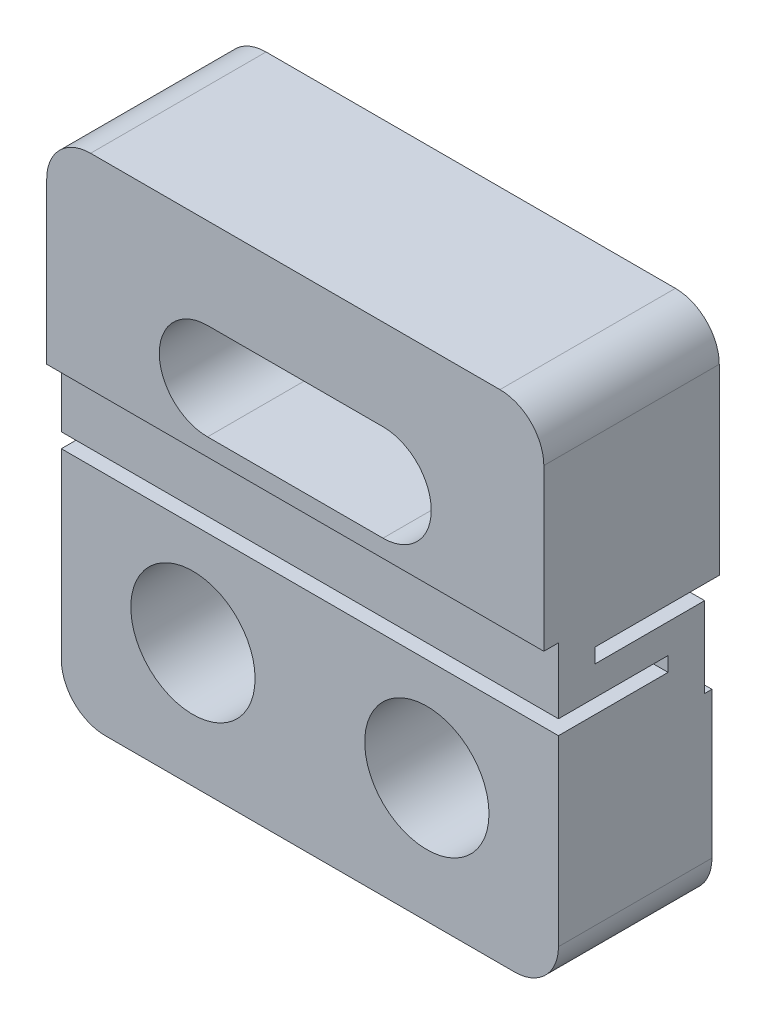
from build123d import *

# Parameters (mm, degrees)
SKETCH1_W           = 34
SKETCH1_H           = 35
BOSS_EXTRUDE1_DEPTH = 12
SKETCH2_R           = 2.1
CUT_EXTRUDE1_DEPTH  = 28.189152249
SKETCH3_W           = 43.383687714
SKETCH3_H           = 21.18675689
CUT_EXTRUDE2_DEPTH  = 1
SKETCH4_W           = 50.621361837
SKETCH4_H           = 17.880513978
CUT_EXTRUDE3_DEPTH  = 0.5
CUT_EXTRUDE4_DEPTH  = 1
SKETCH6_R           = 4.25
CUT_EXTRUDE5_DEPTH  = 6.5
SKETCH7_W           = 35.621240015
SKETCH7_H           = 1
CUT_EXTRUDE6_DEPTH  = 7.5
SKETCH8_W           = 34
SKETCH8_H           = 1
CUT_EXTRUDE7_DEPTH  = 7.5
FILLET1_R           = 3


with BuildPart() as part:
    # Sketch1 → Boss-Extrude1 (new body)
    with BuildSketch(Plane.XY):
        Rectangle(SKETCH1_W, SKETCH1_H)
    extrude(amount=BOSS_EXTRUDE1_DEPTH)

    # Sketch2 → Cut-Extrude1 (cut, through all)
    with BuildSketch(Plane.XY.offset(12)):
        with Locations((-8, -9)):
            Circle(SKETCH2_R)
        with Locations((8, -9)):
            Circle(SKETCH2_R)
        with BuildLine():
            Line((-6, 11.3), (6, 11.3))
            ThreePointArc((6, 11.3), (9.3, 8), (6, 4.7))
            Line((6, 4.7), (-6, 4.7))
            ThreePointArc((-6, 4.7), (-9.3, 8), (-6, 11.3))
        make_face()
    extrude(amount=-CUT_EXTRUDE1_DEPTH, mode=Mode.SUBTRACT)

    # Sketch3 → Cut-Extrude2 (cut)
    with BuildSketch(Plane.XY.offset(12)):
        with Locations((1.327871271, -7.093378445)):
            Rectangle(SKETCH3_W, SKETCH3_H)
    extrude(amount=-CUT_EXTRUDE2_DEPTH, mode=Mode.SUBTRACT)

    # Sketch4 → Cut-Extrude3 (cut)
    with BuildSketch(Plane(origin=(0, 0, 0), x_dir=(-1, 0, 0), z_dir=(0, 0, -1))):
        with Locations((0.547748923, -13.440256989)):
            Rectangle(SKETCH4_W, SKETCH4_H)
    extrude(amount=-CUT_EXTRUDE3_DEPTH, mode=Mode.SUBTRACT)

    # Sketch5 → Cut-Extrude4 (cut)
    with BuildSketch(Plane(origin=(0, 0, 0), x_dir=(-1, 0, 0), z_dir=(0, 0, -1))):
        Polygon((-23.912611607, 2), (26.337975431, 2), (17, -4.5), (-17, -4.5), align=None)
    extrude(amount=-CUT_EXTRUDE4_DEPTH, mode=Mode.SUBTRACT)

    # Sketch6 → Cut-Extrude5 (cut)
    with BuildSketch(Plane.XY.offset(11)):
        with Locations((8, -9)):
            Circle(SKETCH6_R)
        with Locations((-8, -9)):
            Circle(SKETCH6_R)
    extrude(amount=-CUT_EXTRUDE5_DEPTH, mode=Mode.SUBTRACT)

    # Sketch7 → Cut-Extrude6 (cut)
    with BuildSketch(Plane(origin=(0, 0, 1), x_dir=(-1, 0, 0), z_dir=(0, 0, -1))):
        with Locations((-0.810620008, 1.5)):
            Rectangle(SKETCH7_W, SKETCH7_H)
    extrude(amount=-CUT_EXTRUDE6_DEPTH, mode=Mode.SUBTRACT)

    # Sketch8 → Cut-Extrude7 (cut)
    with BuildSketch(Plane.XY.offset(11)):
        with Locations((0, -1.5)):
            Rectangle(SKETCH8_W, SKETCH8_H)
    extrude(amount=-CUT_EXTRUDE7_DEPTH, mode=Mode.SUBTRACT)

    # Fillet1
    fillet1_edges = [part.edges().sort_by_distance(p)[0] for p in [
        (17, -17.5, 5.75),
        (-17, -17.5, 5.75),
        (-17, 17.5, 6),
        (17, 17.5, 6),
    ]]
    fillet(fillet1_edges, radius=FILLET1_R)


solid = part.part
